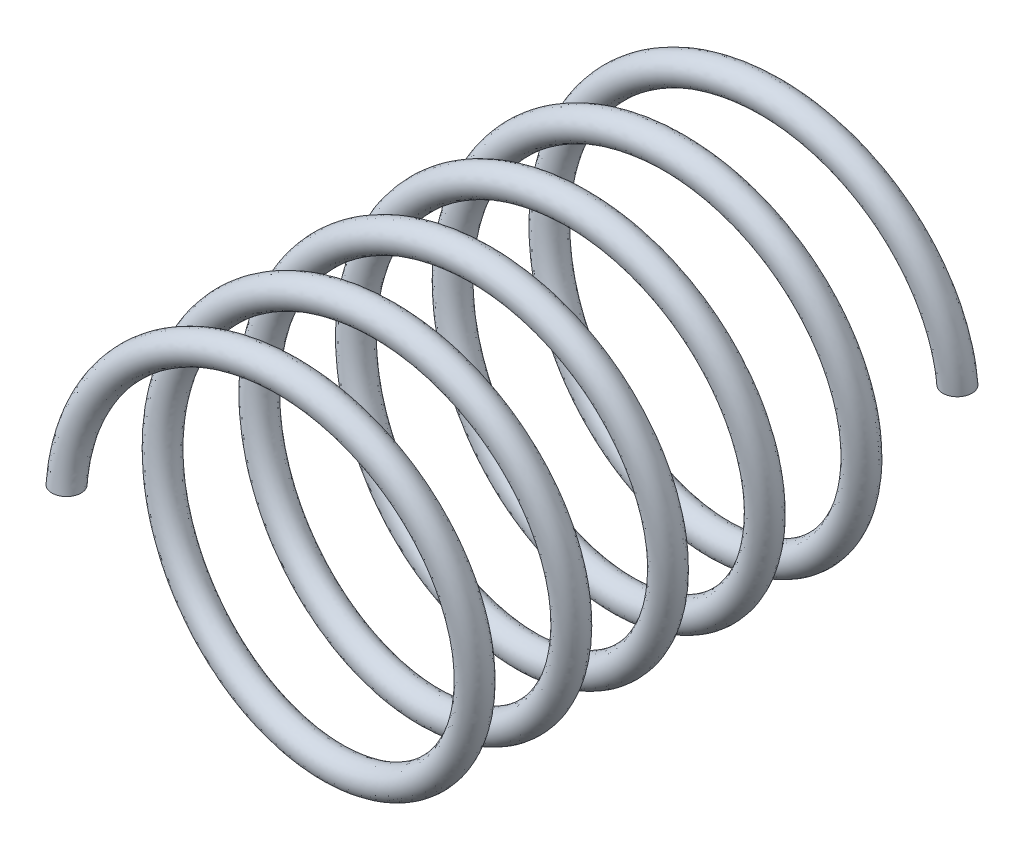
SolidWorks part; units mm, degrees
ref_plane "Front Plane" through (0, 0, 0) normal (0, 0, 1) x (1, 0, 0)
ref_plane "Top Plane" through (0, 0, 0) normal (0, 1, 0) x (1, 0, 0)
ref_plane "Right Plane" through (0, 0, 0) normal (1, 0, 0) x (0, 0, -1)
sketch "Sketch1" plane through (0, 0, 0) normal (0, 0, 1) x (1, 0, 0)
  circle A0 centre (0, 0) radius 30
  dimension "D1" = 60
curve "Helix/Spiral1" pitch 14.95 height 82.225 turns 5.5
sketch "Sketch2" plane through (0, 0, 0) normal (0, 1, 0) x (1, 0, 0)
  circle A0 centre (27.75, 0) radius 2.25
sweep "Sweep1" add profiles "Sketch2" path "Helix/Spiral1"
